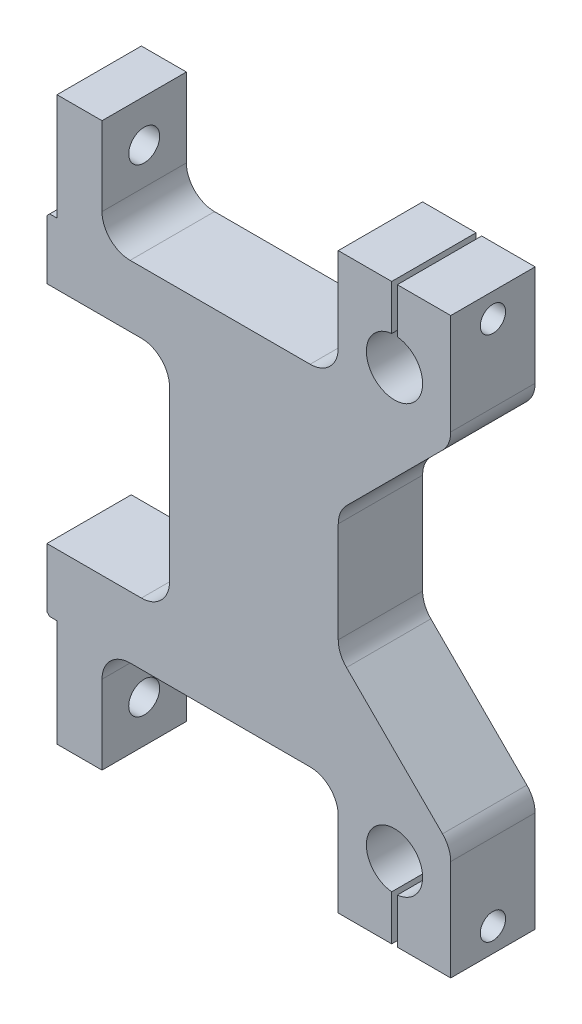
SolidWorks part; units mm, degrees
ref_plane "Front Plane" through (0, 0, 0) normal (0, 0, 1) x (1, 0, 0)
ref_plane "Top Plane" through (0, 0, 0) normal (0, 1, 0) x (1, 0, 0)
ref_plane "Right Plane" through (0, 0, 0) normal (1, 0, 0) x (0, 0, -1)
sketch "Sketch1" plane through (0, 0, 0) normal (0, 1, 0) x (1, 0, 0)
  line L1 (0, 0) -> (72, 0)
  line L2 (0, 0) -> (0, 45)
  line L3 (0, 45) -> (10, 45)
  line L4 (72, 0) -> (72, 15)
  line L7 (72, 15) -> (10, 15)
  line L8 (10, 45) -> (10, 15)
  dimension "D1" = 15
  dimension "D2" = 45
  dimension "D3" = 10
  dimension "D4" = 72
extrude "Boss-Extrude1" add sketch "Sketch1" along normal blind 40
sketch "Sketch2" plane through (0, 0, 0) normal (0, 0, 1) x (1, 0, 0)
  line L0 (0, 40) -> (72, 40) construction
  line L1 (0, 0) -> (52, 0)
  line L2 (0, 0) -> (0, 20)
  line L3 (0, 20) -> (52, 20)
  line L4 (52, 0) -> (52, 20)
  line L5 (72, 40) -> (72, 0) construction
  dimension "D1" = 20
  dimension "D2" = 20
extrude "Cut-Extrude1" cut sketch "Sketch2" against normal blind 56
sketch "Sketch3" plane through (0, 0, 0) normal (0, 0, 1) x (1, 0, 0)
  line L0 (72, 40) -> (72, 0) construction
  line L1 (52, 0) -> (72, 0) construction
  circle A0 centre (62, 13) radius 5
  dimension "D2" = 13
  dimension "D3" = 10
  dimension "D1" = 10
extrude "Cut-Extrude2" cut sketch "Sketch3" against normal blind 56
chamfer "Chamfer1" distance 20 angle 45 1 edges at (72, 40, -7.5)
sketch "Sketch4" plane through (0, 0, 0) normal (0, 0, 1) x (1, 0, 0)
  line L0 (0, 40) -> (52, 40) construction
  line L1 (22, 40) -> (52, 40)
  line L2 (22, 40) -> (22, 51)
  line L3 (22, 51) -> (52, 51)
  line L4 (52, 40) -> (52, 51)
  dimension "D1" = 11
  dimension "D2" = 0
  dimension "D3" = 30
extrude "Boss-Extrude2" add sketch "Sketch4" against normal up to surface (15 mm away) up to face at (67, 13, -15)
sketch "Sketch5" plane through (0, 0, 0) normal (0, 0, 1) x (1, 0, 0)
  line L0 (22, 51) -> (52, 51)
  line L1 (72, 20) -> (72, 0) construction
  line L3 (52, 0) -> (52, 20) construction
  line L5 (0, 40) -> (0, 20) construction
  line L7 (22, 51) -> (22, 40) construction
  line L8 (52, 40) -> (52, 51) construction
  line L16 (22, 62) -> (22, 51)
  line L17 (52, 51) -> (52, 62)
  line L18 (20, 51) -> (50020, 51) construction
  line L19 (0, 62) -> (22, 62)
  line L20 (0, 62) -> (0, 82)
  line L21 (52, 82) -> (0, 82)
  line L22 (52, 102) -> (52, 82)
  line L23 (72, 82) -> (52, 62)
  line L24 (72, 82) -> (72, 102)
  line L25 (52, 102) -> (72, 102)
  circle A0 centre (62, 13) radius 5 construction
  circle A2 centre (62, 89) radius 5
extrude "Boss-Extrude3" add sketch "Sketch5" against normal up to surface (15 mm away) up to face at (67, 13, -15)
sketch "Sketch6" plane through (0, 0, 0) normal (-1, 0, 0) x (0, 0, 1)
  line L0 (0, 51) -> (-50000, 51) construction
  line L1 (0, 62) -> (0, 40) construction
  line L2 (-45, 40) -> (0, 40) construction
  line L3 (-45, 40) -> (-45, 20) construction
  line L4 (-45, 20) -> (0, 20) construction
  line L5 (0, 40) -> (0, 20) construction
  line L6 (-45, 40) -> (0, 40)
  line L7 (-45, 40) -> (-45, 20)
  line L8 (-45, 20) -> (0, 20)
  line L9 (0, 40) -> (0, 20)
  line L10 (0, 62) -> (0, 82)
  line L11 (-45, 82) -> (0, 82)
  line L12 (-45, 62) -> (-45, 82)
  line L13 (-45, 62) -> (0, 62)
  point P4 (0, 51)
extrude "Boss-Extrude4" add sketch "Sketch6" against normal up to surface (10 mm away) up to face at (10, 30, -30)
sketch "Sketch8" plane through (0, 0, 0) normal (-1, 0, 0) x (0, 0, 1)
  line L0 (0, 51) -> (-50000, 51) construction
  line L1 (0, 62) -> (0, 40) construction
  line L2 (-45, 82) -> (-45, 62) construction
  line L3 (2.0615, 31) -> (-45, 31)
  line L4 (2.0615, 31) -> (2.0615, 71)
  line L5 (2.0615, 71) -> (-45, 71)
  line L6 (-45, 31) -> (-45, 71)
  line L7 (2.0615, 31) -> (-45, 71) construction
  line L8 (2.0615, 71) -> (-45, 31) construction
  point P4 (0, 51)
  point P5 (-21.4693, 51)
  dimension "D1" = 40
extrude "Cut-Extrude3" cut sketch "Sketch8" against normal up to surface (22 mm away) up to face at (22, 51, -9.375)
sketch "Sketch9" plane through (10, 0, 0) normal (1, 0, 0) x (0, 0, -1)
  line L0 (0, 51) -> (50000, 51) construction
  line L1 (0, 40) -> (0, 62) construction
  line L2 (0, 82) -> (0, 102) construction
  line L3 (45, 82) -> (0, 82)
  line L4 (45, 82) -> (45, 101)
  line L5 (45, 101) -> (0, 101)
  line L6 (0, 82) -> (0, 101)
  line L7 (45, 1) -> (0, 1)
  line L8 (0, 20) -> (0, 1)
  line L9 (45, 20) -> (0, 20)
  line L10 (45, 20) -> (45, 1)
  point P4 (0, 51)
  dimension "D1" = 100
extrude "Boss-Extrude5" add sketch "Sketch9" against normal blind 8
sketch "Sketch11" plane through (10, 0, 0) normal (1, 0, 0) x (0, 0, -1)
  line L0 (0, 51) -> (50000, 51) construction
  line L1 (0, 40) -> (0, 62) construction
  line L2 (0, 20) -> (0, 0) construction
  circle A0 centre (7.5, 93.5) radius 2.75
  circle A1 centre (7.5, 8.5) radius 2.75
  point P4 (0, 51)
  dimension "D1" = 5.5
  dimension "D2" = 85
  dimension "D3" = 7.5
extrude "Cut-Extrude4" cut sketch "Sketch11" against normal blind 37
sketch "Sketch12" plane through (72, 0, 0) normal (1, 0, 0) x (0, 0, -1)
  line L0 (0, 51) -> (50000, 51) construction
  line L1 (0, 40) -> (0, 62) construction
  line L2 (0, 1) -> (45, 1) construction
  line L3 (45, 101) -> (15, 101)
  line L4 (45, 101) -> (45, 1)
  line L5 (45, 1) -> (15, 1)
  line L6 (15, 101) -> (15, 1)
  line L7 (15, 102) -> (15, 82) construction
  point P4 (0, 51)
extrude "Cut-Extrude5" cut sketch "Sketch12" against normal blind 112
sketch "Sketch13" plane through (0, 0, 0) normal (0, 0, 1) x (1, 0, 0)
  line L0 (2, 20) -> (0, 20) construction
  line L1 (0, 82) -> (0.2, 82)
  line L2 (0, 82) -> (0, 20)
  line L3 (0, 20) -> (0.2, 20)
  line L4 (0.2, 82) -> (0.2, 20)
  dimension "D1" = 0.2
extrude "Cut-Extrude6" cut sketch "Sketch13" against normal blind 112
chamfer "Chamfer2" distance 0.5 angle 45 2 edges at (0.2, 82, -7.5) (0.2, 20, -7.5)
sketch "Sketch14" plane through (0, 0, 0) normal (0, 0, 1) x (1, 0, 0)
  line L0 (62, 89) -> (50062, 89) construction
  line L1 (62, 13) -> (50062, 13) construction
  line L3 (62, 89) -> (62, -49911) construction
  line L4 (22, 51) -> (50022, 51) construction
  line L5 (22, 71) -> (22, 31) construction
  line L6 (52, 0) -> (72, 0) construction
  line L7 (61.5, 9.4429) -> (62.5, 9.4429)
  line L8 (61.5, 9.4429) -> (61.5, 0)
  line L9 (61.5, 0) -> (62.5, 0)
  line L10 (62.5, 9.4429) -> (62.5, 0)
  line L11 (61.5, 9.4429) -> (62.5, 0) construction
  line L12 (61.5, 0) -> (62.5, 9.4429) construction
  line L13 (61.5, 102) -> (62.5, 102)
  line L14 (61.5, 92.5571) -> (61.5, 102)
  line L15 (61.5, 92.5571) -> (62.5, 92.5571)
  line L16 (62.5, 92.5571) -> (62.5, 102)
  point P12 (22, 51)
  point P13 (62, 4.7215)
  dimension "D1" = 1
extrude "Cut-Extrude7" cut sketch "Sketch14" against normal blind 29
sketch "Sketch15" plane through (72, 0, 0) normal (1, 0, 0) x (0, 0, -1)
  line L0 (0, 51) -> (50000, 51) construction
  line L1 (0, 40) -> (0, 62) construction
  line L2 (7.5, 102) -> (7.5, -49898) construction
  line L3 (15, 102) -> (0, 102) construction
  circle A0 centre (7.5, 97.75) radius 2.25
  circle A1 centre (7.5, 4.25) radius 2.25
  point P4 (0, 51)
  point P9 (7.5, 102)
  dimension "D1" = 4.5
  dimension "D2" = 93.5
extrude "Cut-Extrude8" cut sketch "Sketch15" against normal up to surface (9.5 mm away) up to face at (62.5, 97.9875, -7.5)
hole_wizard "M4 Tapped Hole1" positions "3DSketch1" profile "Sketch16" tap size "M4" standard "Gb"
sketch3d "3DSketch1"
  line L0 (62.5, 97.75, -7.5) -> (72, 97.75, -7.5) construction
  point P0 (61.5, 97.75, -7.5)
  dimension "D1" = 0
cosmetic thread "Cosmetic thread 1" parameters "D2"=4
sketch "Sketch16" plane through (61.5, 97.75, -7.5) normal (0, 1, 0) x (0, 0, -1)
  line L0 (0, 0) -> (0, 9.5)
  line L1 (0, 9.5) -> (1.65, 9.5)
  line L2 (1.65, 9.5) -> (1.65, 0)
  line L5 (1.65, 0) -> (0, 0)
  line L11 (0, -6.35) -> (0, 107.95) construction
  dimension "通孔螺纹孔钻头直径" = 3.3
  dimension "通孔螺纹孔钻头深度" = 9.5
hole_wizard "M4 Tapped Hole2" positions "3DSketch2" profile "Sketch17" tap size "M4" standard "Gb"
sketch3d "3DSketch2"
  line L0 (62.5, 4.25, -7.5) -> (72, 4.25, -7.5) construction
  point P0 (61.5, 4.25, -7.5)
  dimension "D1" = 0
cosmetic thread "Cosmetic thread 2" parameters "D2"=4
sketch "Sketch17" plane through (61.5, 4.25, -7.5) normal (0, 1, 0) x (0, 0, -1)
  line L0 (0, 0) -> (0, 9.5)
  line L1 (0, 9.5) -> (1.65, 9.5)
  line L2 (1.65, 9.5) -> (1.65, 0)
  line L5 (1.65, 0) -> (0, 0)
  line L11 (0, -6.35) -> (0, 107.95) construction
  dimension "通孔螺纹孔钻头直径" = 3.3
  dimension "通孔螺纹孔钻头深度" = 9.5
fillet "Fillet1" radius 5 10 edges at (72, 20, -7.5) (72, 82, -7.5) (52, 62, -7.5) (52, 40, -7.5) (52, 82, -7.5) (10, 82, -7.5) (22, 71, -7.5) (22, 31, -7.5) (10, 20, -7.5) (52, 20, -7.5)
